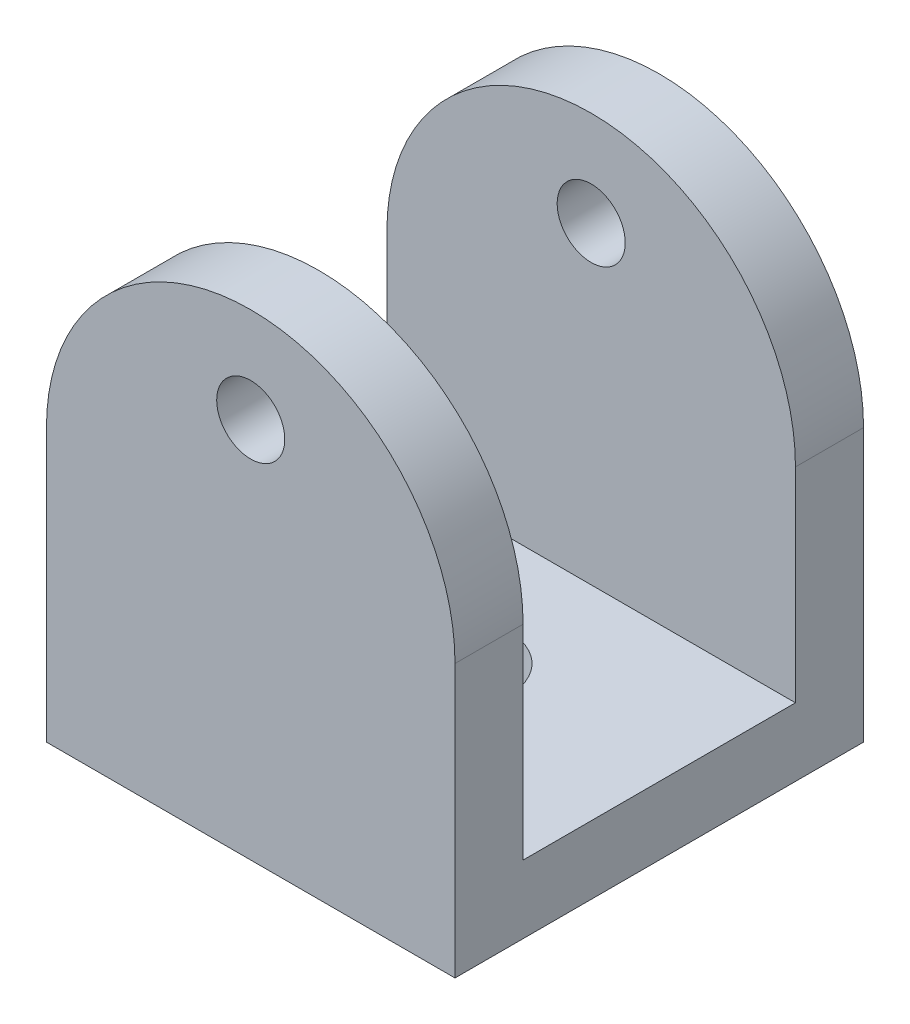
from build123d import *

# Parameters (mm, degrees)
SKETCH_1_W          = 30
SKETCH_1_H          = 40
EXTRUDE_1_DEPTH     = 30
SKETCH_4_W          = 20
SKETCH_4_H          = 35
CUT_EXTRUDE_1_DEPTH = 40
CUT_EXTRUDE_2_DEPTH = 40
SKETCH_6_R          = 2.5
CUT_EXTRUDE_3_DEPTH = 40
SKETCH_7_R          = 4
CUT_EXTRUDE_4_DEPTH = 40


with BuildPart() as part:
    # 草图1 → 凸台-拉伸1 (new body)
    with BuildSketch(Plane.XY):
        with Locations((15, 20)):
            Rectangle(SKETCH_1_W, SKETCH_1_H)
    extrude(amount=EXTRUDE_1_DEPTH)

    # 草图4 → 切除-拉伸1 (cut)
    with BuildSketch(Plane(origin=(30, 0, 0), x_dir=(0, 0, -1), z_dir=(1, 0, 0))):
        with Locations((-15, 22.5)):
            Rectangle(SKETCH_4_W, SKETCH_4_H)
    extrude(amount=-CUT_EXTRUDE_1_DEPTH, mode=Mode.SUBTRACT)

    # 草图5 → 切除-拉伸2 (cut)
    with BuildSketch(Plane(origin=(0, 0, 0), x_dir=(-1, 0, 0), z_dir=(0, 0, -1))):
        with BuildLine():
            Line((-30, 20), (-30, 40))
            Line((-30, 40), (0, 40))
            Line((0, 40), (0, 20))
            ThreePointArc((0, 20), (-15, 35), (-30, 20))
        make_face()
    extrude(amount=-CUT_EXTRUDE_2_DEPTH, mode=Mode.SUBTRACT)

    # 草图6 → 切除-拉伸3 (cut)
    with BuildSketch(Plane(origin=(0, 0, 0), x_dir=(-1, 0, 0), z_dir=(0, 0, -1))):
        with Locations((-15, 28)):
            Circle(SKETCH_6_R)
    extrude(amount=-CUT_EXTRUDE_3_DEPTH, mode=Mode.SUBTRACT)

    # 草图7 → 切除-拉伸4 (cut)
    with BuildSketch(Plane.XZ):
        with Locations(Location((15, 15, 0), (0, 0, 270))):
            Circle(SKETCH_7_R)
    extrude(amount=-CUT_EXTRUDE_4_DEPTH, mode=Mode.SUBTRACT)


solid = part.part
